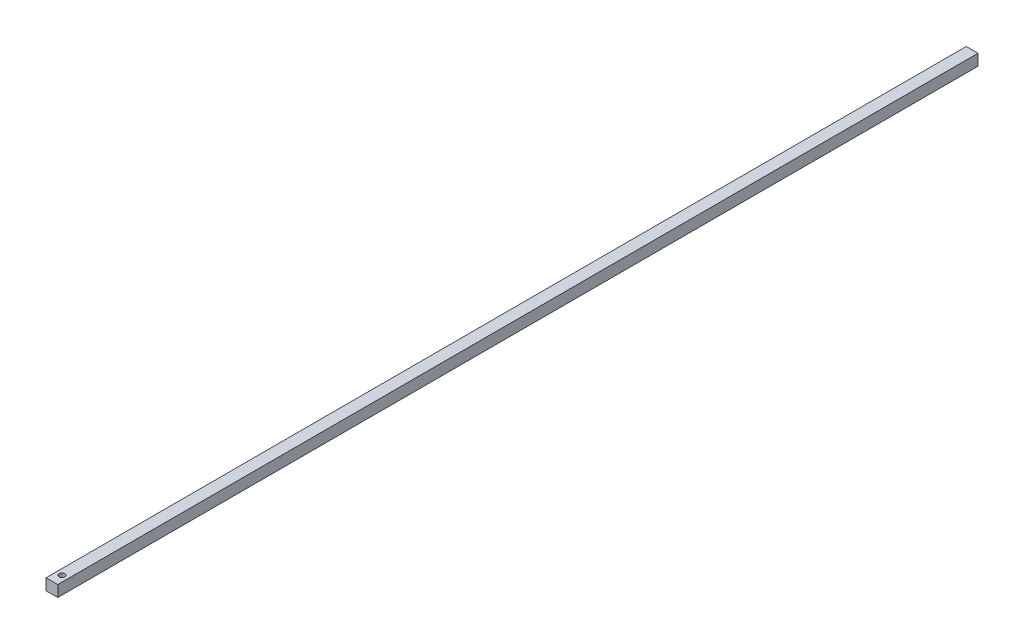
from build123d import *

# Parameters (mm, degrees)
SKETCH_1_W          = 23
SKETCH_1_H          = 22
EXTRUDE_1_DEPTH     = 900
SKETCH_2_R          = 5.5
CUT_EXTRUDE_1_DEPTH = 9
CUT_EXTRUDE_2_REACH = 902.167
SKETCH_3_R          = 3.5


with BuildPart() as part:
    # 草图1 → 凸台-拉伸1 (new, symmetric)
    with BuildSketch(Plane.XY):
        Rectangle(SKETCH_1_W, SKETCH_1_H)
    extrude(amount=EXTRUDE_1_DEPTH, both=True)

    # 草图2 → 切除-拉伸1 (cut)
    with BuildSketch(Plane(origin=(0, 11, 0), x_dir=(1, 0, 0), z_dir=(0, 1, 0))):
        with Locations(Location((0, -880, 0), (0, 0, 180))):
            Circle(SKETCH_2_R)
    extrude(amount=-CUT_EXTRUDE_1_DEPTH, mode=Mode.SUBTRACT)

    # 草图3 → 切除-拉伸2 (cut, up to next)
    with BuildSketch(Plane(origin=(0, 2, 0), x_dir=(1, 0, 0), z_dir=(0, 1, 0)), mode=Mode.PRIVATE) as cut_extrude_2_sk1:
        with Locations(Location((0, -880, 0), (0, 0, 180))):
            Circle(SKETCH_3_R)
    cut_extrude_2_tool1 = extrude(cut_extrude_2_sk1.sketch, amount=-CUT_EXTRUDE_2_REACH, mode=Mode.PRIVATE) & part.part
    add(cut_extrude_2_tool1.solids().sort_by_distance((0, 2, 880))[0], mode=Mode.SUBTRACT)


solid = part.part
